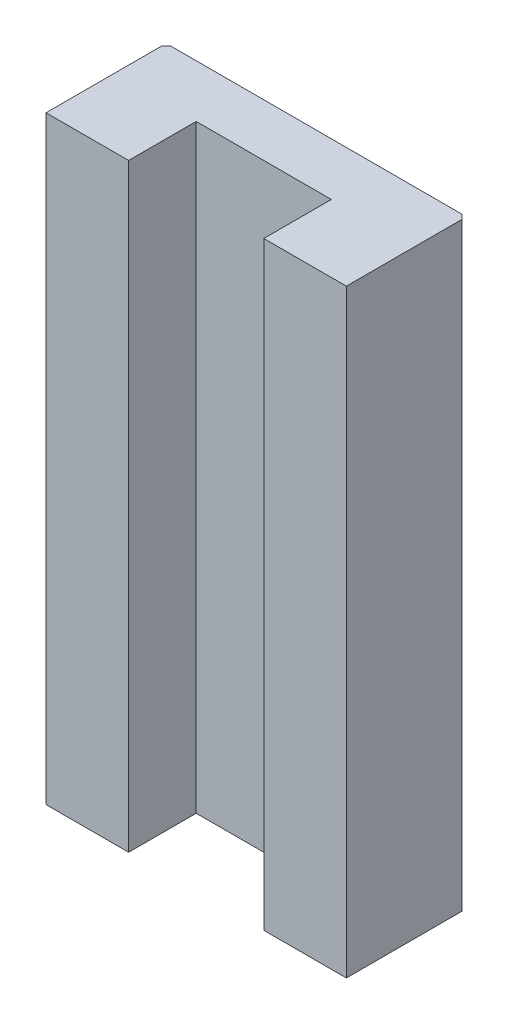
from build123d import *

# Parameters (mm, degrees)
SKETCH1_W             = 20
SKETCH1_H             = 8
BOSS_EXTRUDE1_DEPTH   = 39.9
SKETCH2_W             = 9
SKETCH2_H             = 9
CUT_EXTRUDE1_DEPTH    = 42.328077623
CHAMFER1_SIZE         = 0.3
SKETCH3_R             = 0.5930201
CUT_EXTRUDE2_DEPTH    = 3
SKETCH4_R             = 0.6
CUT_EXTRUDE3_DEPTH    = 4.5
M3_TAPPED_HOLE1_D     = 2.5
M3_TAPPED_HOLE1_DEPTH = 5
M3_TAPPED_HOLE1_TIP   = 0.751075774


with BuildPart() as part:
    # Sketch1 → Boss-Extrude1 (new body)
    with BuildSketch(Plane(origin=(0, 0, 0), x_dir=(1, 0, 0), z_dir=(0, 1, 0))):
        Rectangle(SKETCH1_W, SKETCH1_H)
    extrude(amount=BOSS_EXTRUDE1_DEPTH)

    # Sketch2 → Cut-Extrude1 (cut, through all)
    with BuildSketch(Plane(origin=(0, 39.9, 0), x_dir=(1, 0, 0), z_dir=(0, 1, 0))):
        with Locations((0, -4)):
            Rectangle(SKETCH2_W, SKETCH2_H)
    extrude(amount=-CUT_EXTRUDE1_DEPTH, mode=Mode.SUBTRACT)

    # Chamfer1
    chamfer1_edges = [part.edges().sort_by_distance(p)[0] for p in [
        (-10, 19.95, -4),
        (10, 19.95, -4),
    ]]
    chamfer(chamfer1_edges, length=CHAMFER1_SIZE)

    # Sketch3 → Cut-Extrude2 (cut)
    with BuildSketch(Plane(origin=(0, 0, -4), x_dir=(-1, 0, 0), z_dir=(0, 0, -1))):
        with Locations((-7.5, 27.95)):
            Circle(SKETCH3_R)
        with Locations(Location((7.5, 27.95, 0), (0, 0, 180))):
            Circle(SKETCH3_R)
        with Locations((7.5, 11.95)):
            Circle(SKETCH3_R)
        with Locations(Location((-7.5, 11.95, 0), (0, 0, 180))):
            Circle(SKETCH3_R)
    extrude(amount=-CUT_EXTRUDE2_DEPTH, mode=Mode.SUBTRACT)

    # Sketch4 → Cut-Extrude3 (cut)
    with BuildSketch(Plane.XZ):
        with Locations(Location((0, -2.2, 0), (0, 0, 270))):
            Circle(SKETCH4_R)
    extrude(amount=-CUT_EXTRUDE3_DEPTH, mode=Mode.SUBTRACT)

    # M3 Tapped Hole1
    with Locations(Plane(origin=(7.5, 11.95, -4), x_dir=(-1, 0, 0), z_dir=(0, 0, -1))):
        with Locations((0, 0), (15, 0), (15, 16), (0, 16)):
            Hole(M3_TAPPED_HOLE1_D / 2, depth=M3_TAPPED_HOLE1_DEPTH)
            with Locations((0, 0, -(M3_TAPPED_HOLE1_DEPTH + M3_TAPPED_HOLE1_TIP / 2))):  # 118° drill point
                Cone(0, M3_TAPPED_HOLE1_D / 2, M3_TAPPED_HOLE1_TIP, mode=Mode.SUBTRACT)


solid = part.part
